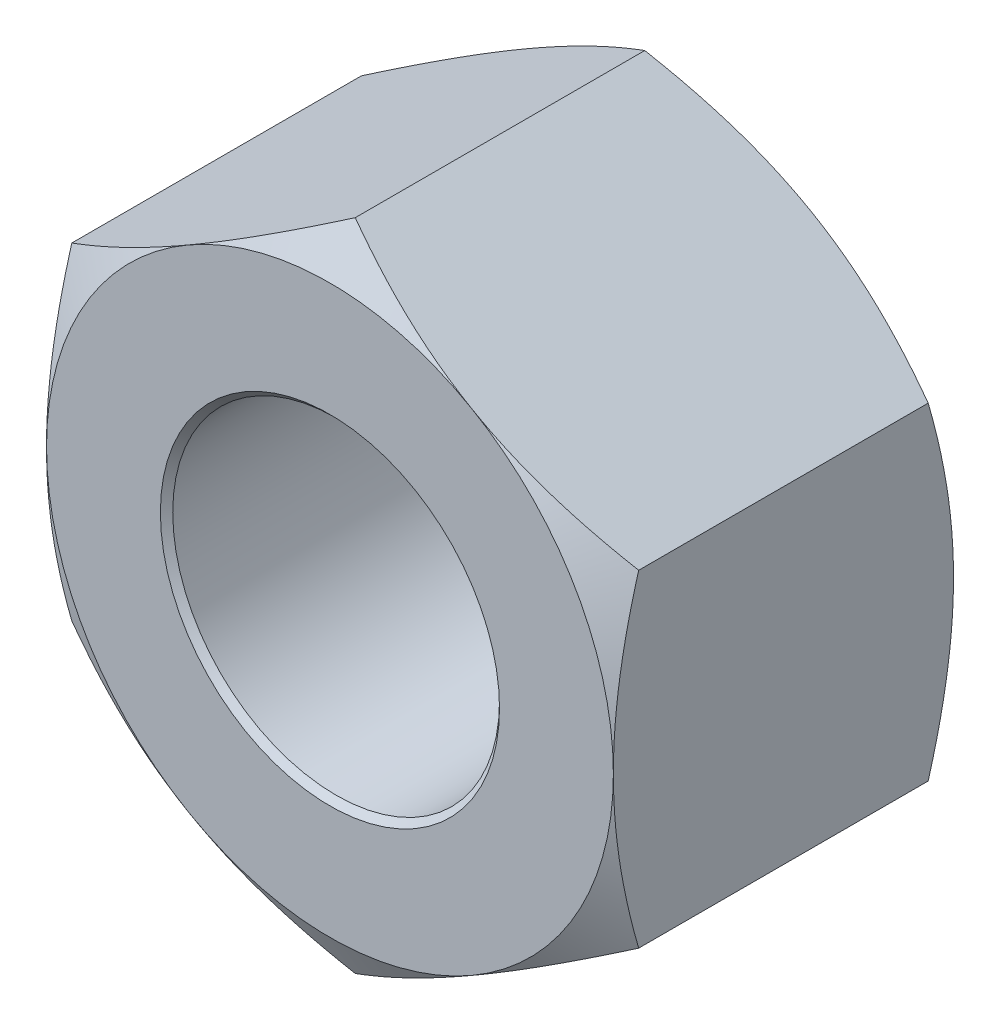
from build123d import *

# Parameters (mm, degrees)
SKETCH_1_R          = 5.188125
EXTRUDE_652_DEPTH   = 10.8
SKETCH_2_OUTSIDE_W  = 89.934
SKETCH_2_OUTSIDE_H  = 92.718
SKETCH_2_OUTSIDE_R  = 9
CUT_EXTRUDE_1_DEPTH = 18.482562741
CUT_EXTRUDE_1_DRAFT = -60
SKETCH_3_OUTSIDE_W  = 89.934
SKETCH_3_OUTSIDE_H  = 92.718
SKETCH_3_OUTSIDE_R  = 9
CUT_EXTRUDE_2_DEPTH = 18.482562741
CUT_EXTRUDE_2_DRAFT = -60
CHAMFER_1_SIZE      = 0.196428571


with BuildPart() as part:
    # 草图1 → Extrude 652 (new body)
    with BuildSketch(Plane.XY):
        Polygon((0, 10.392304845), (-9, 5.196152423), (-9, -5.196152423), (0, -10.392304845), (9, -5.196152423), (9, 5.196152423), align=None)
        with Locations(Location((0, 0, 0), (0, 0, 180))):
            Circle(SKETCH_1_R, mode=Mode.SUBTRACT)
    extrude(amount=EXTRUDE_652_DEPTH)


with BuildPart() as cut_extrude_1_tool:
    # 草图2 outside → 切除-拉伸1 (with draft: the straight prism first)
    with BuildSketch(Plane(origin=(0, 0, 0), x_dir=(-1, 0, 0), z_dir=(0, 0, -1))):
        Rectangle(SKETCH_2_OUTSIDE_W, SKETCH_2_OUTSIDE_H)
        Circle(SKETCH_2_OUTSIDE_R, mode=Mode.SUBTRACT)
    extrude(amount=-CUT_EXTRUDE_1_DEPTH)
    # 切除-拉伸1: the draft: its side faces are tilted about the plane it starts from
    cut_extrude_1_sides = [cut_extrude_1_tool.faces().sort_by_distance(p)[0] for p in [
        (0, -46.359, 9.241281371),
        (-44.967, 0, 9.241281371),
        (0, 46.359, 9.241281371),
        (44.967, 0, 9.241281371),
        (9, 0, 9.241281371),
    ]]
    draft(cut_extrude_1_sides, Plane(origin=(0, 0, 0), x_dir=(-1, 0, 0), z_dir=(0, 0, -1)), CUT_EXTRUDE_1_DRAFT)


with BuildPart() as part_1:
    add(part.part)

    # 切除-拉伸1: cut by cut_extrude_1_tool
    add(cut_extrude_1_tool.part, mode=Mode.SUBTRACT)


with BuildPart() as cut_extrude_2_tool:
    # 草图3 outside → 切除-拉伸2 (with draft: the straight prism first)
    with BuildSketch(Plane.XY.offset(10.8)):
        Rectangle(SKETCH_3_OUTSIDE_W, SKETCH_3_OUTSIDE_H)
        Circle(SKETCH_3_OUTSIDE_R, mode=Mode.SUBTRACT)
    extrude(amount=-CUT_EXTRUDE_2_DEPTH)
    # 切除-拉伸2: the draft: its side faces are tilted about the plane it starts from
    cut_extrude_2_sides = [cut_extrude_2_tool.faces().sort_by_distance(p)[0] for p in [
        (0, -46.359, 1.558718629),
        (44.967, 0, 1.558718629),
        (0, 46.359, 1.558718629),
        (-44.967, 0, 1.558718629),
        (-9, 0, 1.558718629),
    ]]
    draft(cut_extrude_2_sides, Plane.XY.offset(10.8), CUT_EXTRUDE_2_DRAFT)


with BuildPart() as part_2:
    add(part_1.part)

    # 切除-拉伸2: cut by cut_extrude_2_tool
    add(cut_extrude_2_tool.part, mode=Mode.SUBTRACT)

    # 倒角1
    chamfer_1_edges = [part_2.edges().sort_by_distance(p)[0] for p in [
        (5.188125, 0, 0),
        (5.188125, 0, 10.8),
    ]]
    chamfer(chamfer_1_edges, length=CHAMFER_1_SIZE)


solid = part_2.part
